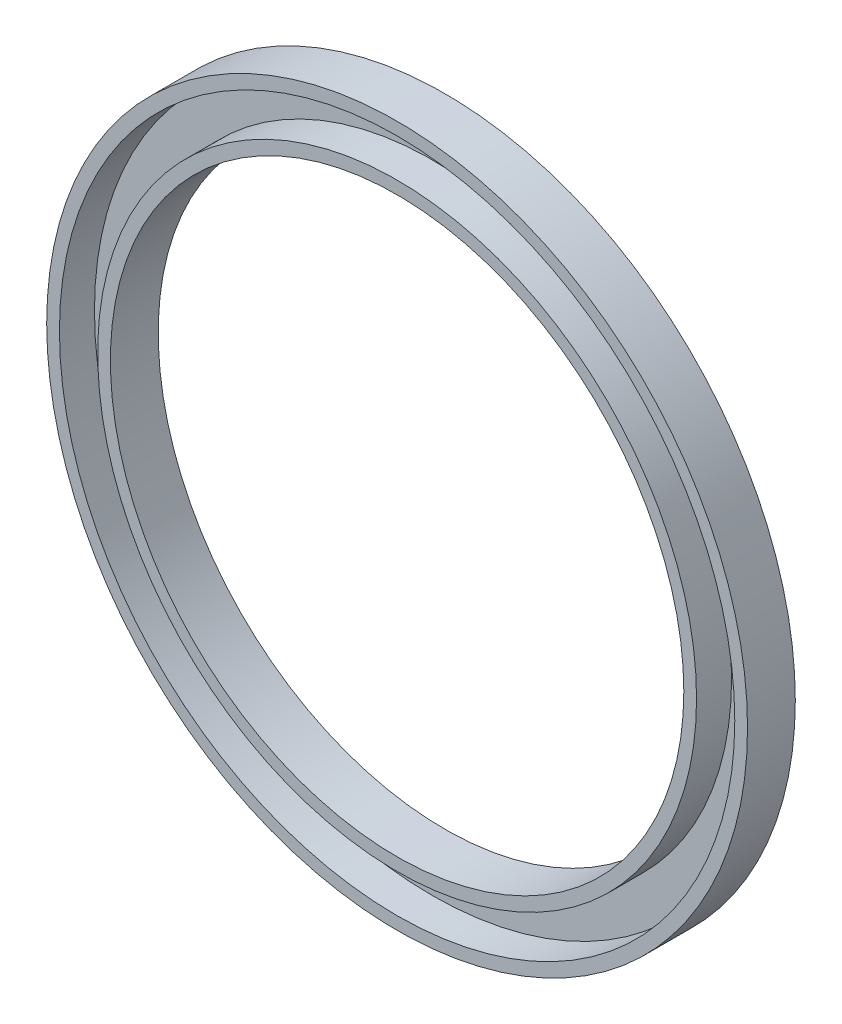
SolidWorks part; units mm, degrees
material "工业胶板"
ref_plane "Front Plane" through (0, 0, 0) normal (0, 0, 1) x (1, 0, 0)
ref_plane "Top Plane" through (0, 0, 0) normal (0, 1, 0) x (1, 0, 0)
ref_plane "Right Plane" through (0, 0, 0) normal (1, 0, 0) x (0, 0, -1)
sketch "Sketch1" plane through (0, 0, 0) normal (0, 0, 1) x (1, 0, 0)
  circle A0 centre (0, 0) radius 110
  circle A1 centre (0, 0) radius 90
  dimension "D1" = 220
  dimension "D2" = 180
extrude "Boss-Extrude1" add sketch "Sketch1" along normal blind 15
shell "Shell1" thickness 4
